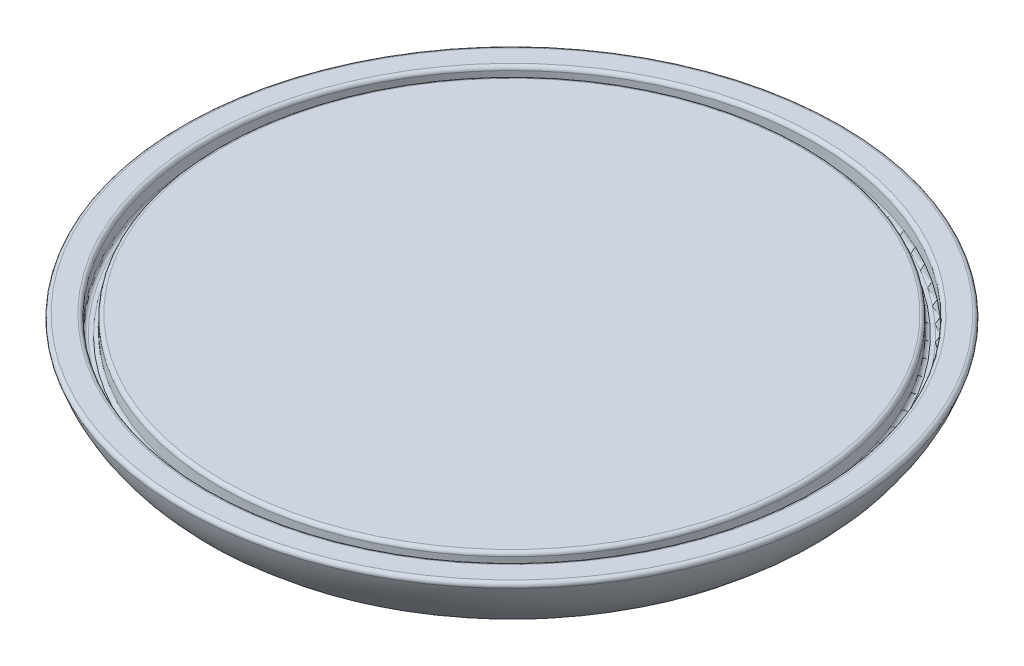
SolidWorks part; units mm, degrees
material "铁"
ref_plane "Front Plane" through (0, 0, 0) normal (0, 0, 1) x (1, 0, 0)
ref_plane "Top Plane" through (0, 0, 0) normal (0, 1, 0) x (1, 0, 0)
ref_plane "Right Plane" through (0, 0, 0) normal (1, 0, 0) x (0, 0, -1)
sketch "Sketch 1" plane through (0, 0, 0) normal (0, 0, 1) x (1, 0, 0)
  line L0 (0, 0) -> (0, 4.0733) construction
  line L1 (-2, -0.4) -> (-6.1086, -0.4)
  line L3 (-8.8654, 1.8) -> (-8.35, 1.8)
  line L4 (-8.25, 1.7) -> (-8.25, 1.4)
  line L5 (-8.15, 1.3) -> (-8.05, 1.3)
  line L6 (-7.95, 1.4) -> (-7.95, 1.7)
  line L7 (-7.85, 1.8) -> (0, 1.8)
  line L8 (0, 1.8) -> (0, 0.4)
  line L9 (0, 0.4) -> (-2, 0.4)
  line L10 (-2, 0.4) -> (-2, -0.4)
  arc A0 (-8.9605, 1.669) -> (-6.1086, -0.4) centre (-6.1086, 2.6) ccw
  arc A1 (-8.9605, 1.669) -> (-8.8654, 1.8) centre (-8.8654, 1.7) cw
  arc A2 (-8.35, 1.8) -> (-8.25, 1.7) centre (-8.35, 1.7) cw
  arc A3 (-8.25, 1.4) -> (-8.15, 1.3) centre (-8.15, 1.4) ccw
  arc A4 (-8.05, 1.3) -> (-7.95, 1.4) centre (-8.05, 1.4) ccw
  arc A5 (-7.95, 1.7) -> (-7.85, 1.8) centre (-7.85, 1.7) cw
  point P16 (-9, 1.8)
  point P19 (-8.25, 1.8)
  point P22 (-8.25, 1.3)
  point P25 (-7.95, 1.3)
  dimension "D1" = 4
  dimension "D7" = 2.2
  dimension "D6" = 3
  dimension "D9" = 0.1
  dimension "D2" = 0.8
  dimension "D3" = 18
  dimension "D4" = 0.3
  dimension "D5" = 0.75
  dimension "D8" = 0.5
revolve "Revolve1" add sketch "Sketch 1" angle 360 about L0
